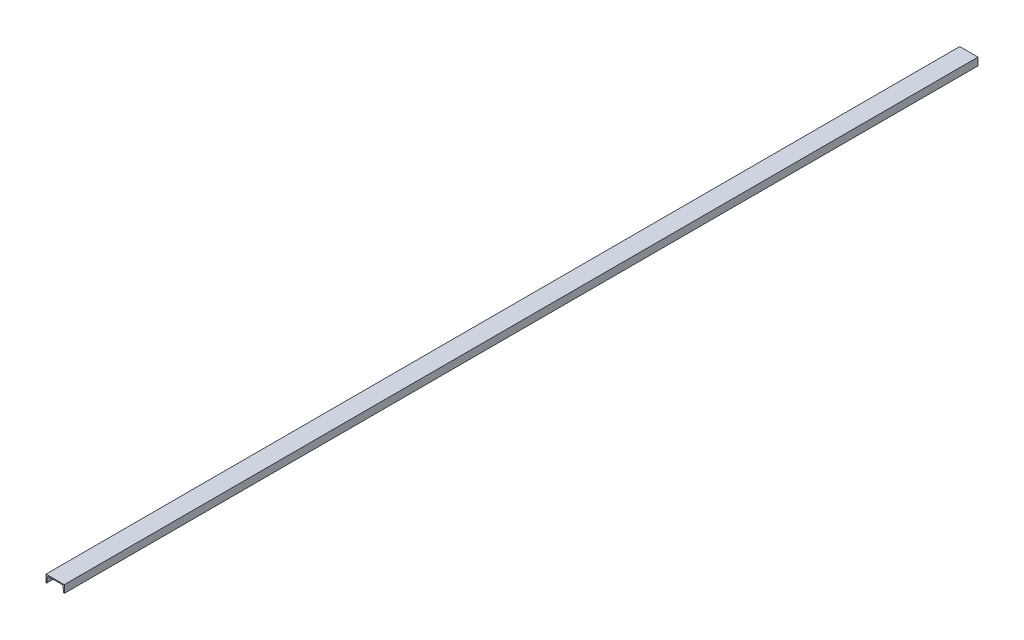
from build123d import *

# Parameters (mm, degrees)
BOSS_EXTRUDE1_DEPTH = 6000


with BuildPart() as part:
    # Sketch1 → Boss-Extrude1 (new body)
    with BuildSketch(Plane.XY):
        with BuildLine():
            Line((0, 0), (0, 50))
            Line((0, 50), (120, 50))
            Line((120, 50), (120, 0))
            Line((120, 0), (117.451472673, 0))
            ThreePointArc((117.451472673, 0), (116.119850629, 0.507759157), (115.464371872, 1.773217267))
            Line((115.464371872, 1.773217267), (111.247290138, 38.723854473))
            ThreePointArc((111.247290138, 38.723854473), (109.608593246, 41.887499748), (106.279538137, 43.156897641))
            Line((106.279538137, 43.156897641), (13.720461863, 43.156897641))
            ThreePointArc((13.720461863, 43.156897641), (10.391406754, 41.887499748), (8.752709862, 38.723854473))
            Line((8.752709862, 38.723854473), (4.535628128, 1.773217267))
            ThreePointArc((4.535628128, 1.773217267), (3.880149371, 0.507759157), (2.548527327, 0))
            Line((2.548527327, 0), (0, 0))
        make_face()
    extrude(amount=BOSS_EXTRUDE1_DEPTH)


solid = part.part
